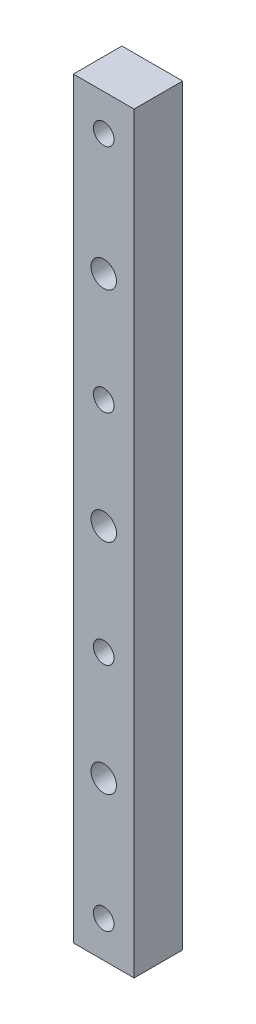
SolidWorks part; units mm, degrees
ref_plane "Front Plane" through (0, 0, 0) normal (0, 0, 1) x (1, 0, 0)
ref_plane "Top Plane" through (0, 0, 0) normal (0, 1, 0) x (1, 0, 0)
ref_plane "Right Plane" through (0, 0, 0) normal (1, 0, 0) x (0, 0, -1)
sketch "Sketch1" plane through (0, 0, 0) normal (0, 0, 1) x (1, 0, 0)
  line L1 (-12.5, -155) -> (12.5, -155)
  line L2 (-12.5, -155) -> (-12.5, 155)
  line L3 (-12.5, 155) -> (12.5, 155)
  line L4 (12.5, -155) -> (12.5, 155)
  line L5 (-12.5, -155) -> (12.5, 155) construction
  line L6 (-12.5, 155) -> (12.5, -155) construction
  point P0 (0, 0)
  dimension "D1" = 25
  dimension "D2" = 310
extrude "Boss-Extrude1" add sketch "Sketch1" along normal blind 20
sketch "Sketch3" plane through (0, 0, 20) normal (0, 0, 1) x (1, 0, 0)
  line L0 (-12.5, 155) -> (-12.5, -155) construction
  line L3 (-12.5, -155) -> (12.5, -155) construction
  circle A1 centre (0, 140) radius 4.25
  circle A2 centre (0, 45) radius 4.25
  circle A3 centre (0, -45) radius 4.25
  circle A4 centre (0, -140) radius 4.25
  dimension "D2" = 8.5
  dimension "D3" = 8.5
  dimension "D4" = 8.5
  dimension "D5" = 8.5
  dimension "D7" = 12.5
  dimension "D8" = 12.5
  dimension "D12" = 95
  dimension "D13" = 90
  dimension "D14" = 95
  dimension "D15" = 15
  dimension "D9" = 12.5
  dimension "D10" = 12.5
extrude "Cut-Extrude1" cut sketch "Sketch3" against normal blind 30
sketch "Sketch5" plane through (0, 0, 0) normal (0, 0, -1) x (-1, 0, 0)
  circle A1 centre (0, 140) radius 6.5
  circle A2 centre (0, 45) radius 6.5
  circle A3 centre (0, -45) radius 6.5
  circle A4 centre (0, -140) radius 6.5
  dimension "D1" = 13
  dimension "D2" = 13
  dimension "D3" = 13
  dimension "D5" = 13
extrude "Cut-Extrude3" cut sketch "Sketch5" against normal blind 10
hole_wizard "M12x1.25 Tapped Hole1" positions "Sketch7" profile "Sketch6" tap size "M12x1.25" standard "Gb"
sketch "Sketch7" plane through (0, 0, 0) normal (0, 0, -1) x (-1, 0, 0)
  line L0 (12.5, -155) -> (-12.5, -155) construction
  point P2 (0, 90)
  point P4 (0, 0)
  point P6 (0, -90)
  dimension "D1" = 65
  dimension "D2" = 90
  dimension "D3" = 90
sketch "Sketch6" plane through (0, 90, 0) normal (1, 0, 0) x (0, 1, 0)
  line L0 (0, 0) -> (0, 33.4045)
  line L1 (0, 33.4045) -> (5.25, 30.25)
  line L2 (5.25, 30.25) -> (5.25, 0)
  line L5 (5.25, 0) -> (0, 0)
  line L10 (0, 33.4045) -> (-5.25, 30.25) construction
  line L11 (0, -6.35) -> (0, 107.95) construction
  dimension "螺纹孔钻头直径" = 10.5
  dimension "螺纹孔钻头深度" = 30.25
  dimension "导头角度" = 118
cosmetic thread "Cosmetic Thread1" parameters "D1"=20, "D2"=12
cosmetic thread "Cosmetic Thread2" parameters "D1"=20, "D2"=12
cosmetic thread "Cosmetic Thread3" parameters "D1"=20, "D2"=12
